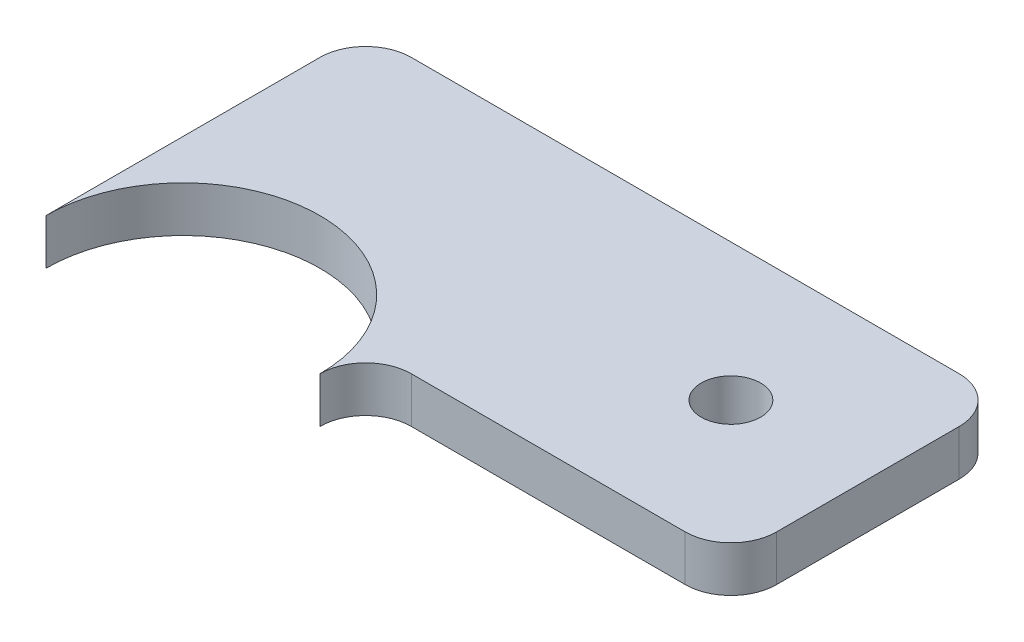
from build123d import *

# Parameters (mm, degrees)
BOSS_EXTRUDE1_DEPTH = 5
FILLET1_R           = 5
SKETCH2_R           = 3.25
CUT_EXTRUDE1_DEPTH  = 5
BOSS_EXTRUDE2_DEPTH = 5


with BuildPart() as part:
    # Sketch1 → Boss-Extrude1 (new body)
    with BuildSketch(Plane(origin=(0, 210, 0), x_dir=(1, 0, 0), z_dir=(0, 1, 0))):
        with BuildLine():
            Line((-15, 0), (-15, 35))
            Line((-15, 35), (55, 35))
            Line((55, 35), (55, 5))
            Line((55, 5), (14.142135624, 5))
            ThreePointArc((14.142135624, 5), (-2.536529681, 14.783978395), (-15, 0))
        make_face()
    extrude(amount=-BOSS_EXTRUDE1_DEPTH)

    # Fillet1
    fillet1_edges = [part.edges().sort_by_distance(p)[0] for p in [
        (-15, 207.5, -35),
        (55, 207.5, -35),
        (55, 207.5, -5),
    ]]
    fillet(fillet1_edges, radius=FILLET1_R)

    # Sketch2 → Cut-Extrude1 (cut)
    with BuildSketch(Plane(origin=(0, 210, 0), x_dir=(1, 0, 0), z_dir=(0, 1, 0))):
        with Locations(Location((40, 20, 0), (0, 0, 270))):
            Circle(SKETCH2_R)
    extrude(amount=-CUT_EXTRUDE1_DEPTH, mode=Mode.SUBTRACT)

    # Sketch3 → Boss-Extrude2 (add)
    with BuildSketch(Plane(origin=(0, 210, 0), x_dir=(1, 0, 0), z_dir=(0, 1, 0))):
        with BuildLine():
            ThreePointArc((15, 0), (16.464466094, 3.535533906), (20, 5))
            Line((20, 5), (14.142135624, 5))
            ThreePointArc((14.142135624, 5), (14.783978395, 2.536529681), (15, 0))
        make_face()
    extrude(amount=-BOSS_EXTRUDE2_DEPTH)


solid = part.part
